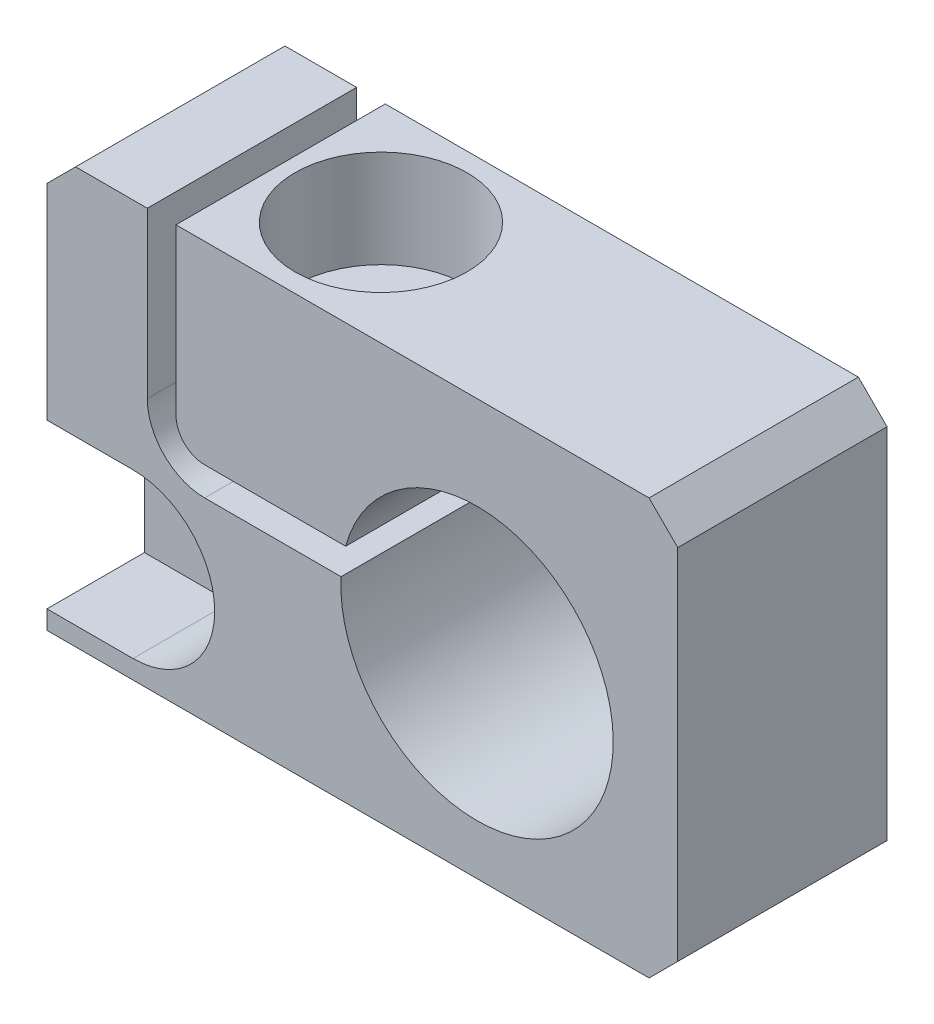
SolidWorks part; units mm, degrees
material "45"
ref_plane "Front Plane" through (0, 0, 0) normal (0, 0, 1) x (1, 0, 0)
ref_plane "Top Plane" through (0, 0, 0) normal (0, 1, 0) x (1, 0, 0)
ref_plane "Right Plane" through (0, 0, 0) normal (1, 0, 0) x (0, 0, -1)
sketch "Sketch1" plane through (0, 0, 0) normal (0, 0, 1) x (1, 0, 0)
  line L1 (-11, -7.25) -> (11, -7.25)
  line L2 (-11, -7.25) -> (-11, 7.25)
  line L3 (-11, 7.25) -> (11, 7.25)
  line L4 (11, -7.25) -> (11, 7.25)
  line L5 (-11, -7.25) -> (11, 7.25) construction
  line L6 (-11, 7.25) -> (11, -7.25) construction
  point P0 (0, 0)
  dimension "D1" = 14.5
  dimension "D2" = 22
extrude "Boss-Extrude1" add sketch "Sketch1" along normal blind 7.3
sketch "Sketch2" plane through (0, 0, 7.3) normal (0, 0, 1) x (1, 0, 0)
  line L0 (-11, -7.25) -> (11, -7.25) construction
  line L1 (11, -7.25) -> (11, 7.25) construction
  circle A0 centre (4, -0.75) radius 4.75
  dimension "D1" = 9.5
  dimension "D3" = 6.5
  dimension "D2" = 7
extrude "Cut-Extrude1" cut sketch "Sketch2" against normal through all
hole_wizard "Ø3.4 (3.4) Diameter Hole1" positions "Sketch4" profile "Sketch3" hole size "Ø3.4" standard "Gb" end condition through all
sketch "Sketch4" plane through (0, 0, 7.3) normal (0, 0, 1) x (1, 0, 0)
  line L4 (-11, 7.25) -> (-11, -7.25) construction
  line L5 (-11, -7.25) -> (11, -7.25) construction
  point P1 (-8, -3.75)
  dimension "D1" = 3.5
  dimension "D3" = 3
sketch "Sketch3" plane through (-8, -3.75, 7.3) normal (1, 0, 0) x (0, -1, 0)
  line L0 (0, 0) -> (0, 7.3)
  line L1 (0, 7.3) -> (1.7, 7.3)
  line L2 (1.7, 7.3) -> (1.7, 0)
  line L5 (1.7, 0) -> (0, 0)
  line L11 (0, -6.35) -> (0, 107.95) construction
  dimension "通孔孔直径" = 3.4
  dimension "通孔孔深度" = 7.3
sketch "Sketch5" plane through (0, 0, 7.3) normal (0, 0, 1) x (1, 0, 0)
  line L1 (7.5, -0.5) -> (-7.5, -0.5)
  line L2 (7.5, -0.5) -> (7.5, 0.5)
  line L3 (7.5, 0.5) -> (-7.5, 0.5)
  line L4 (-7.5, -0.5) -> (-7.5, 0.5)
  line L5 (7.5, -0.5) -> (-7.5, 0.5) construction
  line L6 (7.5, 0.5) -> (-7.5, -0.5) construction
  circle A0 centre (4, -0.75) radius 4.75 construction
  point P0 (0, 0)
  dimension "D1" = 11.5
  dimension "D2" = 1
extrude "Cut-Extrude2" cut sketch "Sketch5" against normal through all
sketch "Sketch6" plane through (0, 0, 7.3) normal (0, 0, 1) x (1, 0, 0)
  line L0 (11, 7.25) -> (-11, 7.25) construction
  line L1 (-7.5, 0.5) -> (-6.5, 0.5)
  line L2 (-7.5, 0.5) -> (-7.5, 7.25)
  line L3 (-7.5, 7.25) -> (-6.5, 7.25)
  line L4 (-6.5, 0.5) -> (-6.5, 7.25)
  dimension "D1" = 1
extrude "Cut-Extrude3" cut sketch "Sketch6" against normal blind 17
fillet "Fillet1" radius 2 1 edges at (-7.5, -0.5, 3.65)
fillet "Fillet2" radius 1 1 edges at (-6.5, 0.5, 3.65)
hole_wizard "M3 Tapped Hole1" positions "Sketch8" profile "Sketch7" tap size "M3" standard "Gb"
sketch "Sketch8" plane through (0, -0.5, 0) normal (0, 1, 0) x (1, 0, 0)
  line L0 (-11, -3.65) -> (-3, -3.65) construction
  line L1 (-11, -7.3) -> (-11, 0) construction
  point P0 (-3, -3.65)
  dimension "D1" = 8
cosmetic thread "Hole cosmetic thread 2" parameters "D2"=3
sketch "Sketch7" plane through (-3, -0.5, 3.65) normal (1, 0, 0) x (0, 0, 1)
  line L0 (0, 0) -> (0, 6.75)
  line L1 (0, 6.75) -> (1.25, 6.75)
  line L2 (1.25, 6.75) -> (1.25, 0)
  line L5 (1.25, 0) -> (0, 0)
  line L11 (0, -6.35) -> (0, 107.95) construction
  dimension "通孔螺纹孔钻头直径" = 2.5
  dimension "通孔螺纹孔钻头深度" = 6.75
hole_wizard "Hole size per socket head cap screw type 3" positions "Sketch12" profile "Sketch11" counterbore size "M3" standard "Gb"
sketch "Sketch12" plane through (0, 7.25, 0) normal (0, 1, 0) x (1, 0, 0)
  line L0 (11, -3.65) -> (-3, -3.65) construction
  line L1 (11, -7.3) -> (11, 0) construction
  point P0 (-3, -3.65)
sketch "Sketch11" plane through (-3, 7.25, 3.65) normal (1, 0, 0) x (0, 0, 1)
  line L0 (0, 0) -> (0, 8.7705)
  line L1 (0, 8.7705) -> (1.7, 7.749)
  line L2 (1.7, 7.749) -> (1.7, 3.4)
  line L3 (1.7, 3.4) -> (3, 3.4)
  line L4 (3, 3.4) -> (3, 0)
  line L5 (3, 0) -> (0, 0)
  line L10 (0, 8.7705) -> (-1.7, 7.749) construction
  line L11 (0, -6.35) -> (0, 107.95) construction
  dimension "孔直径" = 3.4
  dimension "孔深度" = 7.749
  dimension "柱形沉头孔直径" = 6
  dimension "柱形沉头孔深度" = 3.4
  dimension "导头角度" = 118
sketch "Sketch13" plane through (0, 0, 7.3) normal (0, 0, 1) x (1, 0, 0)
  line L0 (-8, -3.75) -> (-13.4758, -3.75) construction
  line L1 (-8, -6.6) -> (-13.4758, -6.6)
  line L2 (-8, -0.9) -> (-13.4758, -0.9)
  arc A0 (-8, -6.6) -> (-8, -0.9) centre (-8, -3.75) ccw
  arc A1 (-13.4758, -0.9) -> (-13.4758, -6.6) centre (-13.4758, -3.75) ccw
  point P3 (-10.7379, -3.75)
  dimension "D1" = 5.7
extrude "Cut-Extrude4" cut sketch "Sketch13" against normal blind 3.4
chamfer "Chamfer1" distance 1 angle 45 3 edges at (11, -7.25, 3.65) (11, 7.25, 3.65) (-11, 7.25, 3.65)
